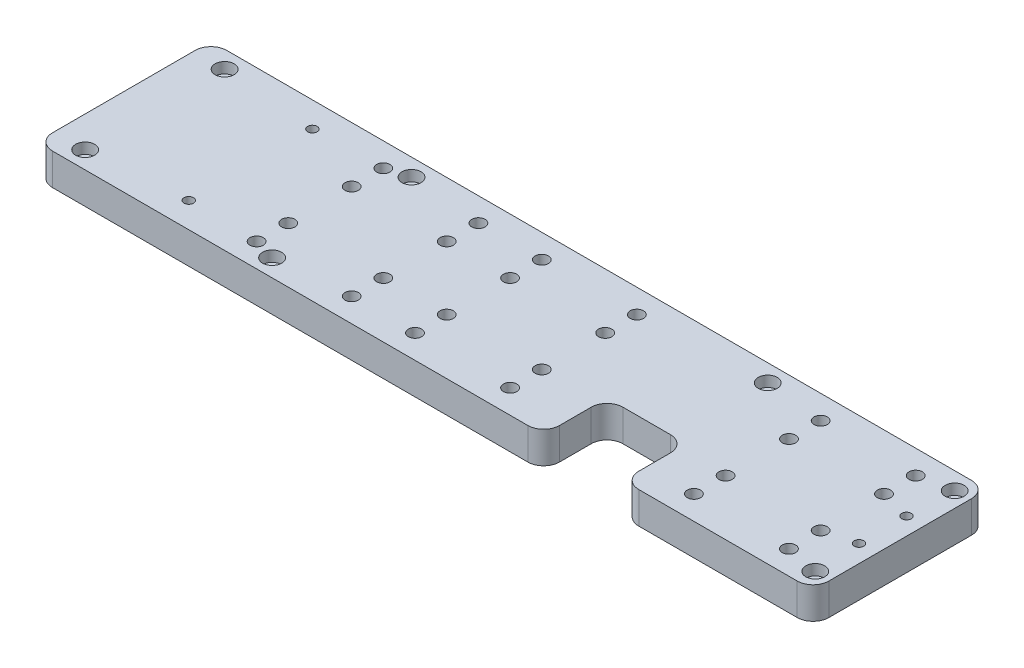
from build123d import *

# Parameters (mm, degrees)
BOSS_EXTRUDE1_DEPTH                                  = 10
CBORE_FOR_M3_HEXAGON_SOCKET_HEAD_CAP_SCR_D           = 3.4
CBORE_FOR_M3_HEXAGON_SOCKET_HEAD_CAP_SCR_DEPTH       = 17
CBORE_FOR_M3_HEXAGON_SOCKET_HEAD_CAP_SCR_CBORE_D     = 6
CBORE_FOR_M3_HEXAGON_SOCKET_HEAD_CAP_SCR_CBORE_DEPTH = 3.4
CBORE_FOR_M3_HEXAGON_SOCKET_HEAD_CAP_SCR_TIP         = 1.021463052
M5_TAPPED_HOLE1_AT_2_COUNT                           = 2
M5_TAPPED_HOLE1_AT_2_PITCH                           = 30
M5_TAPPED_HOLE1_AT_3_COUNT                           = 2
M5_TAPPED_HOLE1_AT_3_PITCH                           = 42.426406871
M5_TAPPED_HOLE1_AT_4_COUNT                           = 2
M5_TAPPED_HOLE1_AT_4_PITCH                           = 10
M5_TAPPED_HOLE1_AT_5_COUNT                           = 2
M5_TAPPED_HOLE1_AT_5_PITCH                           = 31.622776602
M5_TAPPED_HOLE1_AT_6_COUNT                           = 2
M5_TAPPED_HOLE1_AT_6_PITCH                           = 141.223227551
M5_TAPPED_HOLE1_AT_7_COUNT                           = 2
M5_TAPPED_HOLE1_AT_7_PITCH                           = 170.65755184
M5_TAPPED_HOLE1_AT_8_COUNT                           = 2
M5_TAPPED_HOLE1_AT_8_PITCH                           = 138.361844451
M5_TAPPED_HOLE1_AT_9_COUNT                           = 2
M5_TAPPED_HOLE1_AT_9_PITCH                           = 168.300533599
M5_TAPPED_HOLE1_AT_10_COUNT                          = 2
M5_TAPPED_HOLE1_AT_10_PITCH                          = 36.055512755
M5_TAPPED_HOLE1_AT_11_COUNT                          = 2
M5_TAPPED_HOLE1_AT_11_PITCH                          = 20
M5_TAPPED_HOLE1_AT_12_COUNT                          = 2
M5_TAPPED_HOLE1_AT_12_PITCH                          = 139.441744108
M5_TAPPED_HOLE1_AT_13_COUNT                          = 2
M5_TAPPED_HOLE1_AT_13_PITCH                          = 169.18628786
M5_TAPPED_HOLE1_AT_14_COUNT                          = 2
M5_TAPPED_HOLE1_AT_14_PITCH                          = 168
M5_TAPPED_HOLE1_AT_15_COUNT                          = 2
M5_TAPPED_HOLE1_AT_15_PITCH                          = 138
M5_TAPPED_HOLE1_AT_16_COUNT                          = 2
M5_TAPPED_HOLE1_AT_16_PITCH                          = 30
SKETCH6_R                                            = 1.5
CUT_EXTRUDE1_DEPTH                                   = 126.946417178
LPATTERN1_COUNT                                      = 2
LPATTERN1_PITCH                                      = 50


with BuildPart() as part:
    # Sketch1 → Boss-Extrude1 (new body)
    with BuildSketch(Plane(origin=(0, -16.846378111, 0), x_dir=(1, 0, 0), z_dir=(0, 1, 0))):
        with BuildLine():
            Line((67.5, -27.5), (117.5, -27.5))
            ThreePointArc((117.5, -27.5), (121.035533906, -26.035533906), (122.5, -22.5))
            Line((122.5, -22.5), (122.5, 22.5))
            ThreePointArc((122.5, 22.5), (121.035533906, 26.035533906), (117.5, 27.5))
            Line((117.5, 27.5), (-117.5, 27.5))
            ThreePointArc((-117.5, 27.5), (-121.035533906, 26.035533906), (-122.5, 22.5))
            Line((-122.5, 22.5), (-122.5, -22.5))
            ThreePointArc((-122.5, -22.5), (-121.035533906, -26.035533906), (-117.5, -27.5))
            Line((-117.5, -27.5), (32.5, -27.5))
            ThreePointArc((32.5, -27.5), (36.035533906, -26.035533906), (37.5, -22.5))
            Line((37.5, -22.5), (37.5, -12.5))
            ThreePointArc((37.5, -12.5), (38.964466094, -8.964466094), (42.5, -7.5))
            Line((42.5, -7.5), (57.5, -7.5))
            ThreePointArc((57.5, -7.5), (61.035533906, -8.964466094), (62.5, -12.5))
            Line((62.5, -12.5), (62.5, -22.5))
            ThreePointArc((62.5, -22.5), (63.964466094, -26.035533906), (67.5, -27.5))
        make_face()
    extrude(amount=BOSS_EXTRUDE1_DEPTH)

    # CBORE for M3 Hexagon socket head cap screws1
    with Locations(Plane(origin=(0, -6.846378111, 0), x_dir=(1, 0, 0), z_dir=(0, 1, 0))):
        with Locations((117.7, 22), (58.7, 22), (117.7, -22), (-53.7, -22), (-53.7, 22), (-112.7, 22), (-112.7, -22)):
            CounterBoreHole(CBORE_FOR_M3_HEXAGON_SOCKET_HEAD_CAP_SCR_D / 2, CBORE_FOR_M3_HEXAGON_SOCKET_HEAD_CAP_SCR_CBORE_D / 2, CBORE_FOR_M3_HEXAGON_SOCKET_HEAD_CAP_SCR_CBORE_DEPTH, depth=CBORE_FOR_M3_HEXAGON_SOCKET_HEAD_CAP_SCR_DEPTH)
            with Locations((0, 0, -(CBORE_FOR_M3_HEXAGON_SOCKET_HEAD_CAP_SCR_DEPTH + CBORE_FOR_M3_HEXAGON_SOCKET_HEAD_CAP_SCR_TIP / 2))):  # 118° drill point
                Cone(0, CBORE_FOR_M3_HEXAGON_SOCKET_HEAD_CAP_SCR_D / 2, CBORE_FOR_M3_HEXAGON_SOCKET_HEAD_CAP_SCR_TIP, mode=Mode.SUBTRACT)

    # Sketch5 → M5 Tapped Hole1 (revolve, cut)
    with BuildSketch(Plane(origin=(-60.6, -6.846378111, 10), x_dir=(0, 0, 1), z_dir=(1, 0, 0))):
        Polygon((0, 0), (0, 15.2618073), (2.1, 14), (2.1, 0), align=None)
    m5_tapped_hole1 = revolve(axis=Axis((-60.6, -0.496378111, 10), (0, -1, 0)), mode=Mode.SUBTRACT)

    # M5 Tapped Hole1 at 2: M5 Tapped Hole1 ×2
    with Locations(*[(0, 0, -i * M5_TAPPED_HOLE1_AT_2_PITCH) for i in range(1, M5_TAPPED_HOLE1_AT_2_COUNT)]):
        add(m5_tapped_hole1, mode=Mode.SUBTRACT)

    # M5 Tapped Hole1 at 3: M5 Tapped Hole1 ×2
    with Locations(*[Vector(0.7071067811865475, 0, -0.7071067811865476) * (i * M5_TAPPED_HOLE1_AT_3_PITCH) for i in range(1, M5_TAPPED_HOLE1_AT_3_COUNT)]):
        add(m5_tapped_hole1, mode=Mode.SUBTRACT)

    # M5 Tapped Hole1 at 4: M5 Tapped Hole1 ×2
    with Locations(*[(0, 0, i * M5_TAPPED_HOLE1_AT_4_PITCH) for i in range(1, M5_TAPPED_HOLE1_AT_4_COUNT)]):
        add(m5_tapped_hole1, mode=Mode.SUBTRACT)

    # M5 Tapped Hole1 at 5: M5 Tapped Hole1 ×2
    with Locations(*[Vector(0.9486832980505138, 0, 0.3162277660168382) * (i * M5_TAPPED_HOLE1_AT_5_PITCH) for i in range(1, M5_TAPPED_HOLE1_AT_5_COUNT)]):
        add(m5_tapped_hole1, mode=Mode.SUBTRACT)

    # M5 Tapped Hole1 at 6: M5 Tapped Hole1 ×2
    with Locations(*[Vector(0.9771763639228009, 0, -0.21242964433104378) * (i * M5_TAPPED_HOLE1_AT_6_PITCH) for i in range(1, M5_TAPPED_HOLE1_AT_6_COUNT)]):
        add(m5_tapped_hole1, mode=Mode.SUBTRACT)

    # M5 Tapped Hole1 at 7: M5 Tapped Hole1 ×2
    with Locations(*[Vector(0.984427575508482, 0, -0.17579063848365759) * (i * M5_TAPPED_HOLE1_AT_7_PITCH) for i in range(1, M5_TAPPED_HOLE1_AT_7_COUNT)]):
        add(m5_tapped_hole1, mode=Mode.SUBTRACT)

    # M5 Tapped Hole1 at 8: M5 Tapped Hole1 ×2
    with Locations(*[Vector(0.9973847959828921, 0, 0.0722742605784705) * (i * M5_TAPPED_HOLE1_AT_8_PITCH) for i in range(1, M5_TAPPED_HOLE1_AT_8_COUNT)]):
        add(m5_tapped_hole1, mode=Mode.SUBTRACT)

    # M5 Tapped Hole1 at 9: M5 Tapped Hole1 ×2
    with Locations(*[Vector(0.9982332185134931, 0, 0.05941751809182934) * (i * M5_TAPPED_HOLE1_AT_9_PITCH) for i in range(1, M5_TAPPED_HOLE1_AT_9_COUNT)]):
        add(m5_tapped_hole1, mode=Mode.SUBTRACT)

    # M5 Tapped Hole1 at 10: M5 Tapped Hole1 ×2
    with Locations(*[Vector(0.8320502943378436, 0, -0.5547001962252293) * (i * M5_TAPPED_HOLE1_AT_10_PITCH) for i in range(1, M5_TAPPED_HOLE1_AT_10_COUNT)]):
        add(m5_tapped_hole1, mode=Mode.SUBTRACT)

    # M5 Tapped Hole1 at 11: M5 Tapped Hole1 ×2
    with Locations(*[(0, 0, -i * M5_TAPPED_HOLE1_AT_11_PITCH) for i in range(1, M5_TAPPED_HOLE1_AT_11_COUNT)]):
        add(m5_tapped_hole1, mode=Mode.SUBTRACT)

    # M5 Tapped Hole1 at 12: M5 Tapped Hole1 ×2
    with Locations(*[Vector(0.9896605990003554, 0, -0.14342907231889213) * (i * M5_TAPPED_HOLE1_AT_12_PITCH) for i in range(1, M5_TAPPED_HOLE1_AT_12_COUNT)]):
        add(m5_tapped_hole1, mode=Mode.SUBTRACT)

    # M5 Tapped Hole1 at 13: M5 Tapped Hole1 ×2
    with Locations(*[Vector(0.9929882741949438, 0, -0.11821288978511241) * (i * M5_TAPPED_HOLE1_AT_13_PITCH) for i in range(1, M5_TAPPED_HOLE1_AT_13_COUNT)]):
        add(m5_tapped_hole1, mode=Mode.SUBTRACT)

    # M5 Tapped Hole1 at 14: M5 Tapped Hole1 ×2
    with Locations(*[(i * M5_TAPPED_HOLE1_AT_14_PITCH, 0, 0) for i in range(1, M5_TAPPED_HOLE1_AT_14_COUNT)]):
        add(m5_tapped_hole1, mode=Mode.SUBTRACT)

    # M5 Tapped Hole1 at 15: M5 Tapped Hole1 ×2
    with Locations(*[(i * M5_TAPPED_HOLE1_AT_15_PITCH, 0, 0) for i in range(1, M5_TAPPED_HOLE1_AT_15_COUNT)]):
        add(m5_tapped_hole1, mode=Mode.SUBTRACT)

    # M5 Tapped Hole1 at 16: M5 Tapped Hole1 ×2
    with Locations(*[(i * M5_TAPPED_HOLE1_AT_16_PITCH, 0, 0) for i in range(1, M5_TAPPED_HOLE1_AT_16_COUNT)]):
        add(m5_tapped_hole1, mode=Mode.SUBTRACT)

    # Sketch6 → Cut-Extrude1 (cut, through all)
    with BuildSketch(Plane.XZ.offset(16.846378111)):
        with Locations(Location((-82.5, 19.5, 0), (0, 0, 270))):
            Circle(SKETCH6_R)
        with Locations(Location((-82.5, -19.5, 0), (0, 0, 270))):
            Circle(SKETCH6_R)
        with Locations(Location((117, 7.5, 0), (0, 0, 270))):
            Circle(SKETCH6_R)
        with Locations(Location((117, -7.5, 0), (0, 0, 270))):
            Circle(SKETCH6_R)
    extrude(amount=-CUT_EXTRUDE1_DEPTH, mode=Mode.SUBTRACT)

    # LPattern1: M5 Tapped Hole1 ×2
    with Locations(*[(i * LPATTERN1_PITCH, 0, 0) for i in range(1, LPATTERN1_COUNT)]):
        add(m5_tapped_hole1, mode=Mode.SUBTRACT)

    # LPattern1 copy 1 sketch → LPattern1 copy 1 (revolve, cut)
    with BuildSketch(Plane(origin=(-10.6, -6.846378111, -20), x_dir=(0, 0, 1), z_dir=(1, 0, 0))):
        Polygon((0, 0), (0, 15.2618073), (2.1, 14), (2.1, 0), align=None)
    revolve(axis=Axis((-10.6, -0.496378111, -20), (0, -1, 0)), mode=Mode.SUBTRACT)

    # LPattern1 copy 2 sketch → LPattern1 copy 2 (revolve, cut)
    with BuildSketch(Plane(origin=(19.4, -6.846378111, -20), x_dir=(0, 0, 1), z_dir=(1, 0, 0))):
        Polygon((0, 0), (0, 15.2618073), (2.1, 14), (2.1, 0), align=None)
    revolve(axis=Axis((19.4, -0.496378111, -20), (0, -1, 0)), mode=Mode.SUBTRACT)

    # LPattern1 copy 3 sketch → LPattern1 copy 3 (revolve, cut)
    with BuildSketch(Plane(origin=(-10.6, -6.846378111, 20), x_dir=(0, 0, 1), z_dir=(1, 0, 0))):
        Polygon((0, 0), (0, 15.2618073), (2.1, 14), (2.1, 0), align=None)
    revolve(axis=Axis((-10.6, -0.496378111, 20), (0, -1, 0)), mode=Mode.SUBTRACT)

    # LPattern1 copy 4 sketch → LPattern1 copy 4 (revolve, cut)
    with BuildSketch(Plane(origin=(19.4, -6.846378111, 20), x_dir=(0, 0, 1), z_dir=(1, 0, 0))):
        Polygon((0, 0), (0, 15.2618073), (2.1, 14), (2.1, 0), align=None)
    revolve(axis=Axis((19.4, -0.496378111, 20), (0, -1, 0)), mode=Mode.SUBTRACT)

    # LPattern1 copy 5 sketch → LPattern1 copy 5 (revolve, cut)
    with BuildSketch(Plane(origin=(127.4, -6.846378111, -20), x_dir=(0, 0, 1), z_dir=(1, 0, 0))):
        Polygon((0, 0), (0, 15.2618073), (2.1, 14), (2.1, 0), align=None)
    revolve(axis=Axis((127.4, -0.496378111, -20), (0, -1, 0)), mode=Mode.SUBTRACT)

    # LPattern1 copy 6 sketch → LPattern1 copy 6 (revolve, cut)
    with BuildSketch(Plane(origin=(157.4, -6.846378111, -20), x_dir=(0, 0, 1), z_dir=(1, 0, 0))):
        Polygon((0, 0), (0, 15.2618073), (2.1, 14), (2.1, 0), align=None)
    revolve(axis=Axis((157.4, -0.496378111, -20), (0, -1, 0)), mode=Mode.SUBTRACT)

    # LPattern1 copy 7 sketch → LPattern1 copy 7 (revolve, cut)
    with BuildSketch(Plane(origin=(127.4, -6.846378111, 20), x_dir=(0, 0, 1), z_dir=(1, 0, 0))):
        Polygon((0, 0), (0, 15.2618073), (2.1, 14), (2.1, 0), align=None)
    revolve(axis=Axis((127.4, -0.496378111, 20), (0, -1, 0)), mode=Mode.SUBTRACT)

    # LPattern1 copy 8 sketch → LPattern1 copy 8 (revolve, cut)
    with BuildSketch(Plane(origin=(157.403183332, -6.846378111, 20), x_dir=(0, 0, 1), z_dir=(1, 0, 0))):
        Polygon((0, 0), (0, 15.2618073), (2.1, 14), (2.1, 0), align=None)
    revolve(axis=Axis((157.403183332, -0.496378111, 20), (0, -1, 0)), mode=Mode.SUBTRACT)

    # LPattern1 copy 9 sketch → LPattern1 copy 9 (revolve, cut)
    with BuildSketch(Plane(origin=(19.4, -6.846378111, -10), x_dir=(0, 0, 1), z_dir=(1, 0, 0))):
        Polygon((0, 0), (0, 15.2618073), (2.1, 14), (2.1, 0), align=None)
    revolve(axis=Axis((19.4, -0.496378111, -10), (0, -1, 0)), mode=Mode.SUBTRACT)

    # LPattern1 copy 10 sketch → LPattern1 copy 10 (revolve, cut)
    with BuildSketch(Plane(origin=(-10.6, -6.846378111, -10), x_dir=(0, 0, 1), z_dir=(1, 0, 0))):
        Polygon((0, 0), (0, 15.2618073), (2.1, 14), (2.1, 0), align=None)
    revolve(axis=Axis((-10.6, -0.496378111, -10), (0, -1, 0)), mode=Mode.SUBTRACT)

    # LPattern1 copy 11 sketch → LPattern1 copy 11 (revolve, cut)
    with BuildSketch(Plane(origin=(127.4, -6.846378111, -10), x_dir=(0, 0, 1), z_dir=(1, 0, 0))):
        Polygon((0, 0), (0, 15.2618073), (2.1, 14), (2.1, 0), align=None)
    revolve(axis=Axis((127.4, -0.496378111, -10), (0, -1, 0)), mode=Mode.SUBTRACT)

    # LPattern1 copy 12 sketch → LPattern1 copy 12 (revolve, cut)
    with BuildSketch(Plane(origin=(157.4, -6.846378111, -10), x_dir=(0, 0, 1), z_dir=(1, 0, 0))):
        Polygon((0, 0), (0, 15.2618073), (2.1, 14), (2.1, 0), align=None)
    revolve(axis=Axis((157.4, -0.496378111, -10), (0, -1, 0)), mode=Mode.SUBTRACT)

    # LPattern1 copy 13 sketch → LPattern1 copy 13 (revolve, cut)
    with BuildSketch(Plane(origin=(157.4, -6.846378111, 10), x_dir=(0, 0, 1), z_dir=(1, 0, 0))):
        Polygon((0, 0), (0, 15.2618073), (2.1, 14), (2.1, 0), align=None)
    revolve(axis=Axis((157.4, -0.496378111, 10), (0, -1, 0)), mode=Mode.SUBTRACT)

    # LPattern1 copy 14 sketch → LPattern1 copy 14 (revolve, cut)
    with BuildSketch(Plane(origin=(127.4, -6.846378111, 10), x_dir=(0, 0, 1), z_dir=(1, 0, 0))):
        Polygon((0, 0), (0, 15.2618073), (2.1, 14), (2.1, 0), align=None)
    revolve(axis=Axis((127.4, -0.496378111, 10), (0, -1, 0)), mode=Mode.SUBTRACT)

    # LPattern1 copy 15 sketch → LPattern1 copy 15 (revolve, cut)
    with BuildSketch(Plane(origin=(19.4, -6.846378111, 10), x_dir=(0, 0, 1), z_dir=(1, 0, 0))):
        Polygon((0, 0), (0, 15.2618073), (2.1, 14), (2.1, 0), align=None)
    revolve(axis=Axis((19.4, -0.496378111, 10), (0, -1, 0)), mode=Mode.SUBTRACT)


solid = part.part
